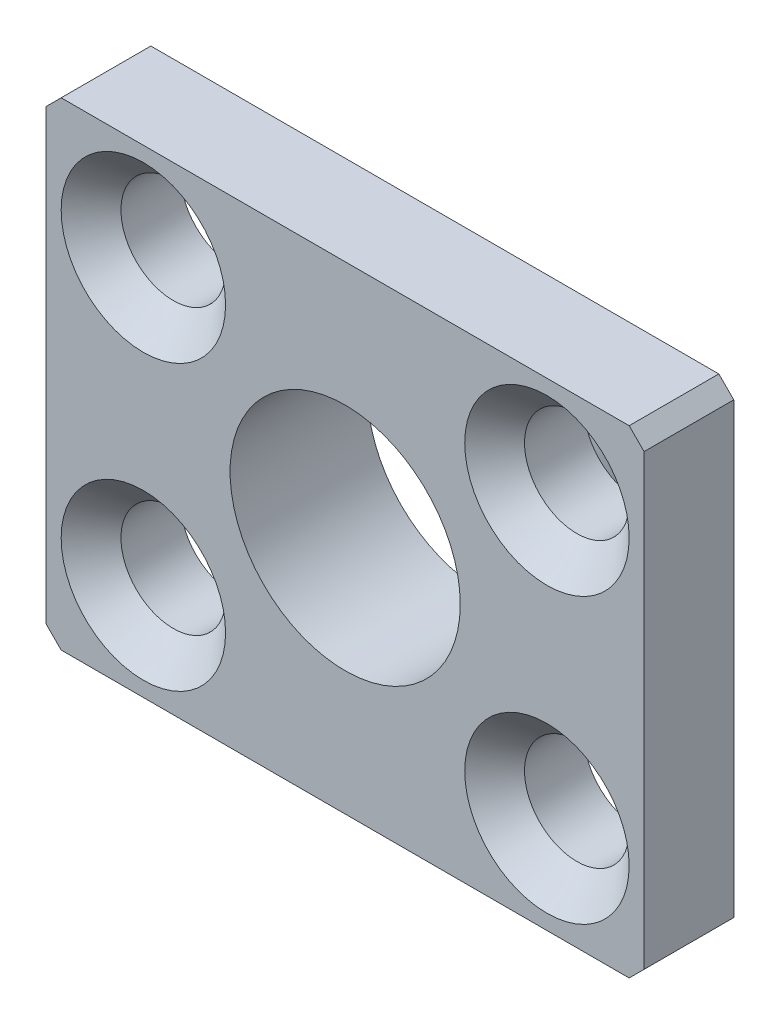
from build123d import *

# Parameters (mm, degrees)
SKETCH1_R           = 5.45
SKETCH1_R_2         = 3.85
BOSS_EXTRUDE1_DEPTH = 1.6
SKETCH2_W           = 20
SKETCH2_H           = 16
SKETCH2_R           = 3.85
SKETCH2_R_2         = 1.75
BOSS_EXTRUDE2_DEPTH = 3
CHAMFER1_SIZE       = 0.3
CHAMFER2_SIZE       = 1
CHAMFER3_SIZE       = 0.5


with BuildPart() as part:
    # Sketch1 → Boss-Extrude1 (new body)
    with BuildSketch(Plane.XY):
        Circle(SKETCH1_R)
        Circle(SKETCH1_R_2, mode=Mode.SUBTRACT)
    extrude(amount=BOSS_EXTRUDE1_DEPTH)

    # Sketch2 → Boss-Extrude2 (add)
    with BuildSketch(Plane.XY.offset(1.6)):
        Rectangle(SKETCH2_W, SKETCH2_H)
        Circle(SKETCH2_R, mode=Mode.SUBTRACT)
        with Locations((-6.75, 4.75)):
            Circle(SKETCH2_R_2, mode=Mode.SUBTRACT)
        with Locations((-6.75, -4.75)):
            Circle(SKETCH2_R_2, mode=Mode.SUBTRACT)
        with Locations((6.75, -4.75)):
            Circle(SKETCH2_R_2, mode=Mode.SUBTRACT)
        with Locations((6.75, 4.75)):
            Circle(SKETCH2_R_2, mode=Mode.SUBTRACT)
    extrude(amount=BOSS_EXTRUDE2_DEPTH)

    # Chamfer1
    chamfer1_edges = [part.edges().sort_by_distance(p)[0] for p in [
        (-5.45, 0, 0),
    ]]
    chamfer(chamfer1_edges, length=CHAMFER1_SIZE)

    # Chamfer2
    chamfer2_edges = [part.edges().sort_by_distance(p)[0] for p in [
        (-8.5, 4.75, 4.6),
        (-8.5, -4.75, 4.6),
        (5, -4.75, 4.6),
        (5, 4.75, 4.6),
    ]]
    chamfer(chamfer2_edges, length=CHAMFER2_SIZE)

    # Chamfer3
    chamfer3_edges = [part.edges().sort_by_distance(p)[0] for p in [
        (10, -8, 3.1),
        (10, 8, 3.1),
        (-10, 8, 3.1),
        (-10, -8, 3.1),
    ]]
    chamfer(chamfer3_edges, length=CHAMFER3_SIZE)


solid = part.part
